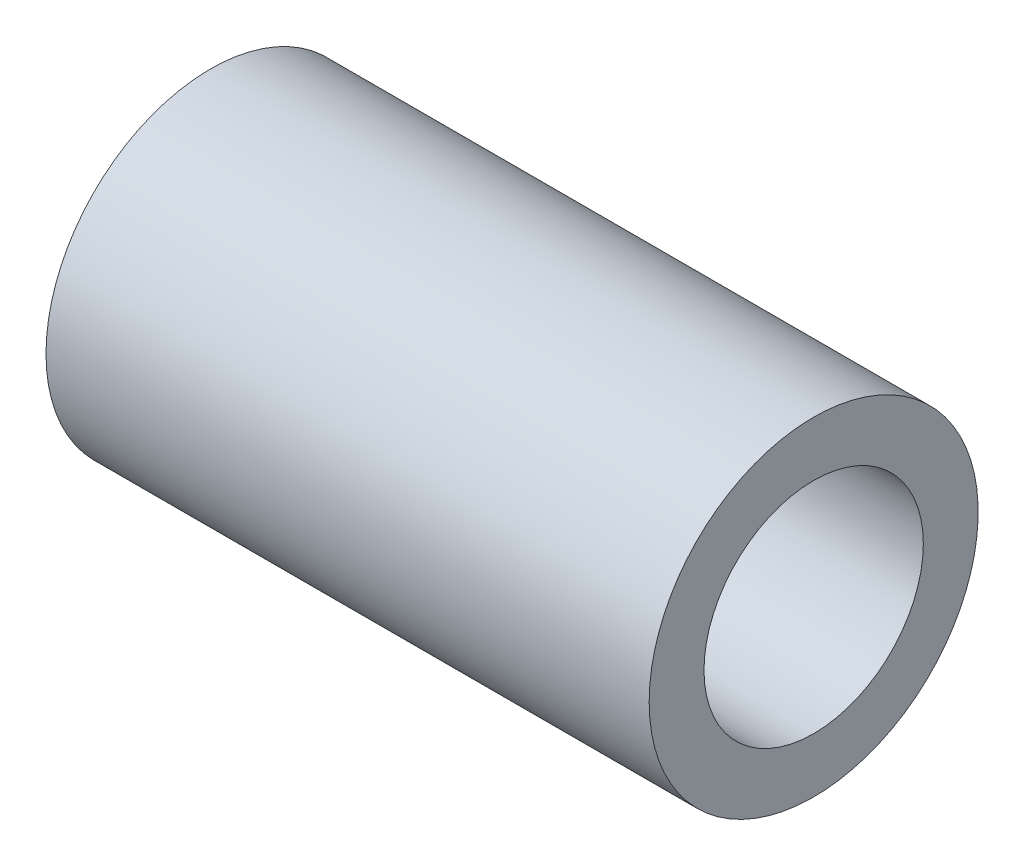
from build123d import *

# Parameters (mm, degrees)
SKETCH_1_W = 22
SKETCH_1_H = 2


with BuildPart() as part:
    # 草图1 → 旋转1 (revolve)
    with BuildSketch(Plane.XY, mode=Mode.PRIVATE) as revolve_1_sk:
        with Locations((11, 5)):
            Rectangle(SKETCH_1_W, SKETCH_1_H)
    revolve(revolve_1_sk.sketch.rotate(Axis((-539.035928085, 0, 0), (1, 0, 0)), 90), axis=Axis((-539.035928085, 0, 0), (1, 0, 0)))


solid = part.part
